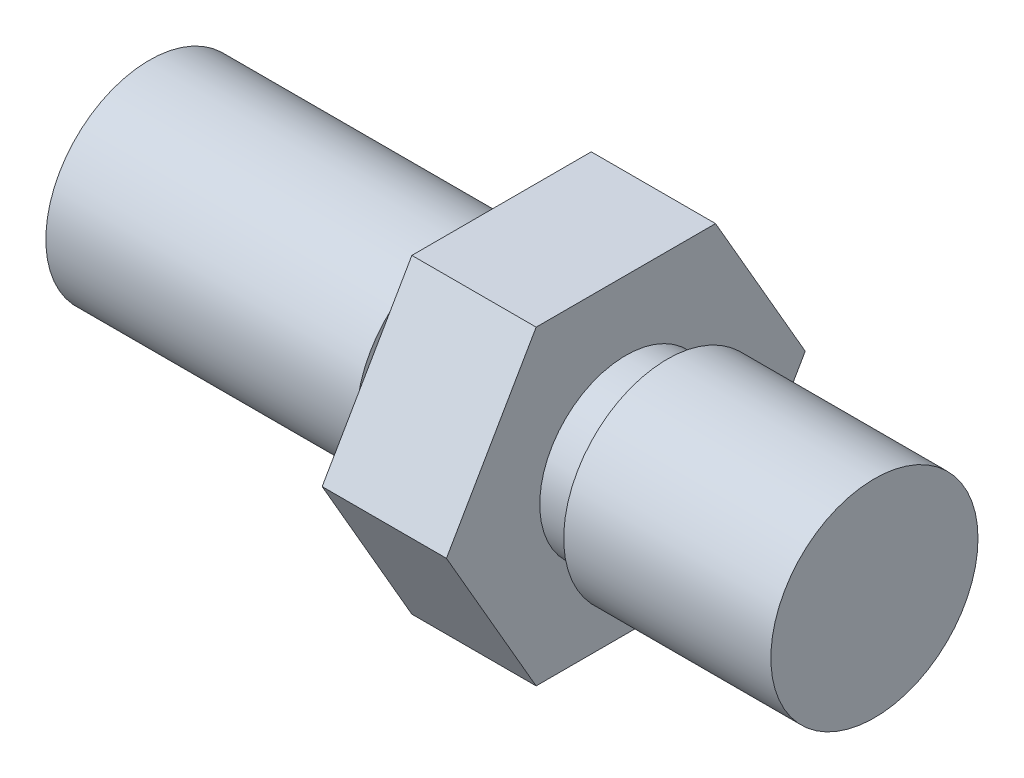
from build123d import *

# Parameters (mm, degrees)
EXTRUDE_1_DEPTH = 6


with BuildPart() as part:
    # 草图1 → 凸台-拉伸1 (new body)
    with BuildSketch(Plane(origin=(8, 0, 0), x_dir=(0, 0, -1), z_dir=(1, 0, 0))):
        Polygon((-8.660254038, 0), (-4.330127019, -7.5), (4.330127019, -7.5), (8.660254038, 0), (4.330127019, 7.5), (-4.330127019, 7.5), align=None)
    extrude(amount=-EXTRUDE_1_DEPTH)

    # 草图2 → 旋转1 (revolve)
    with BuildSketch(Plane.XY, mode=Mode.PRIVATE) as revolve_1_sk:
        Polygon((-15, 5), (-15, 0), (2, 0), (2, 4.157220044), (0, 4.157220044), (0, 5), align=None)
    revolve(revolve_1_sk.sketch.rotate(Axis((-15, 0, 0), (1, 0, 0)), 270), axis=Axis((-15, 0, 0), (1, 0, 0)))

    # 草图3 → 旋转2 (revolve)
    with BuildSketch(Plane.XY, mode=Mode.PRIVATE) as revolve_2_sk:
        Polygon((8, 4.157220044), (8, 0), (20, 0), (20, 5), (10, 5), (10, 4.157220044), align=None)
    revolve(revolve_2_sk.sketch.rotate(Axis((8, 0, 0), (1, 0, 0)), 270), axis=Axis((8, 0, 0), (1, 0, 0)))


solid = part.part
